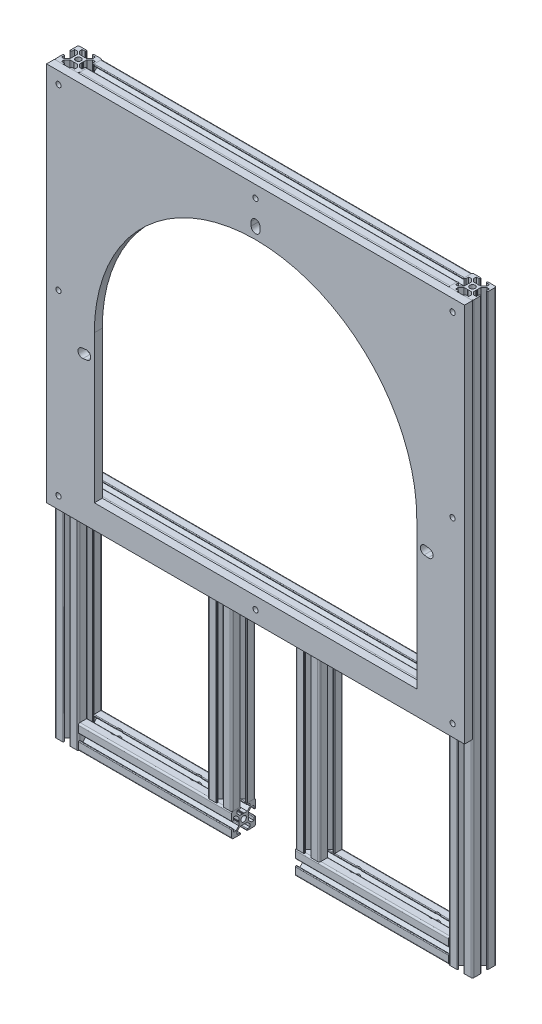
from build123d import *

# Parameters (mm, degrees)
F_30_X_30_X_R2_1_DEPTH      = 722.5
F_30_X_30_X_R2_1_DEPTH_BACK = 15
SKETCH_1_R                  = 3.4
SKETCH_1_ON_SEGMENT_2_R     = 3.4
F_30_X_30_X_R2_1_2_DEPTH    = 737.5
SKETCH_1_ON_SEGMENT_3_R     = 3.4
F_30_X_30_X_R2_1_3_DEPTH    = 497
SKETCH_1_ON_SEGMENT_4_R     = 3.4
F_30_X_30_X_R2_1_4_DEPTH    = 208.5
SKETCH_1_ON_SEGMENT_5_R     = 3.4
F_30_X_30_X_R2_1_5_DEPTH    = 497
SKETCH_1_ON_SEGMENT_6_R     = 3.4
F_30_X_30_X_R2_1_6_DEPTH    = 208.5
SKETCH_1_ON_SEGMENT_7_R     = 3.4
F_30_X_30_X_R2_1_7_DEPTH    = 262
SKETCH_1_ON_SEGMENT_8_R     = 3.4
F_30_X_30_X_R2_1_8_DEPTH    = 262
SKETCH_5_W                  = 525
SKETCH_5_H                  = 477.5
EXTRUDE_1_DEPTH             = 10
CUT_EXTRUDE_1_DEPTH         = 10
SKETCH_7_R                  = 3.25
CUT_EXTRUDE_2_DEPTH         = 10
SKETCH_8_R                  = 5.5
CUT_EXTRUDE_3_DEPTH         = 756.041389594


with BuildPart() as part:
    # 草图1 → 铝型材 30 X 30 X R2(1) (new, two sides: drawn at the far end of the back side and taken through both)
    with BuildSketch(Plane(origin=(-247.5, 367.5, 0), x_dir=(1, 0, 0), z_dir=(0, -1, 0)).offset(-F_30_X_30_X_R2_1_DEPTH_BACK)):
        with BuildLine():
            Line((-15, -4.8), (-15, -13))
            ThreePointArc((-15, -13), (-14.414213562, -14.414213562), (-13, -15))
            Line((-13, -15), (-4.8, -15))
            ThreePointArc((-4.8, -15), (-4.234314575, -14.765685425), (-4, -14.2))
            Line((-4, -14.2), (-4, -13.8))
            ThreePointArc((-4, -13.8), (-4.234314575, -13.234314575), (-4.8, -13))
            Line((-4.8, -13), (-8.25, -13))
            Line((-8.25, -13), (-8.25, -9.664213562))
            Line((-8.25, -9.664213562), (-4.585786438, -6))
            Line((-4.585786438, -6), (-0.653589838, -6))
            ThreePointArc((-0.653589838, -6), (-0.524180316, -5.982962913), (-0.403589838, -5.933012702))
            Line((-0.403589838, -5.933012702), (0, -5.7))
            Line((0, -5.7), (0.403589838, -5.933012702))
            ThreePointArc((0.403589838, -5.933012702), (0.653589838, -6), (0.903589838, -5.933012702))
            Line((0.903589838, -5.933012702), (1.218885629, -5.750976592))
            Line((1.218885629, -5.750976592), (2.5, -6))
            Line((2.5, -6), (4.585786438, -6))
            Line((4.585786438, -6), (8.25, -9.664213562))
            Line((8.25, -9.664213562), (8.25, -13))
            Line((8.25, -13), (4.8, -13))
            ThreePointArc((4.8, -13), (4.234314575, -13.234314575), (4, -13.8))
            Line((4, -13.8), (4, -14.2))
            ThreePointArc((4, -14.2), (4.234314575, -14.765685425), (4.8, -15))
            Line((4.8, -15), (13, -15))
            ThreePointArc((13, -15), (14.414213562, -14.414213562), (15, -13))
            Line((15, -13), (15, -4.8))
            ThreePointArc((15, -4.8), (14.765685425, -4.234314575), (14.2, -4))
            Line((14.2, -4), (13.8, -4))
            ThreePointArc((13.8, -4), (13.234314575, -4.234314575), (13, -4.8))
            Line((13, -4.8), (13, -8.25))
            Line((13, -8.25), (9.664213562, -8.25))
            Line((9.664213562, -8.25), (6, -4.585786438))
            Line((6, -4.585786438), (6, -0.653589838))
            ThreePointArc((6, -0.653589838), (5.982962913, -0.524180316), (5.933012702, -0.403589838))
            Line((5.933012702, -0.403589838), (5.7, 0))
            Line((5.7, 0), (5.933012702, 0.403589838))
            ThreePointArc((5.933012702, 0.403589838), (6, 0.653589838), (5.933012702, 0.903589838))
            Line((5.933012702, 0.903589838), (5.750976592, 1.218885629))
            Line((5.750976592, 1.218885629), (6, 2.5))
            Line((6, 2.5), (6, 4.585786438))
            Line((6, 4.585786438), (9.664213562, 8.25))
            Line((9.664213562, 8.25), (13, 8.25))
            Line((13, 8.25), (13, 4.8))
            ThreePointArc((13, 4.8), (13.234314575, 4.234314575), (13.8, 4))
            Line((13.8, 4), (14.2, 4))
            ThreePointArc((14.2, 4), (14.765685425, 4.234314575), (15, 4.8))
            Line((15, 4.8), (15, 13))
            ThreePointArc((15, 13), (14.414213562, 14.414213562), (13, 15))
            Line((13, 15), (4.8, 15))
            ThreePointArc((4.8, 15), (4.234314575, 14.765685425), (4, 14.2))
            Line((4, 14.2), (4, 13.8))
            ThreePointArc((4, 13.8), (4.234314575, 13.234314575), (4.8, 13))
            Line((4.8, 13), (8.25, 13))
            Line((8.25, 13), (8.25, 9.664213562))
            Line((8.25, 9.664213562), (4.585786438, 6))
            Line((4.585786438, 6), (0.653589838, 6))
            ThreePointArc((0.653589838, 6), (0.524180316, 5.982962913), (0.403589838, 5.933012702))
            Line((0.403589838, 5.933012702), (0, 5.7))
            Line((0, 5.7), (-0.403589838, 5.933012702))
            ThreePointArc((-0.403589838, 5.933012702), (-0.653589838, 6), (-0.903589838, 5.933012702))
            Line((-0.903589838, 5.933012702), (-1.218885629, 5.750976592))
            Line((-1.218885629, 5.750976592), (-2.5, 6))
            Line((-2.5, 6), (-4.585786438, 6))
            Line((-4.585786438, 6), (-8.25, 9.664213562))
            Line((-8.25, 9.664213562), (-8.25, 13))
            Line((-8.25, 13), (-4.8, 13))
            ThreePointArc((-4.8, 13), (-4.234314575, 13.234314575), (-4, 13.8))
            Line((-4, 13.8), (-4, 14.2))
            ThreePointArc((-4, 14.2), (-4.234314575, 14.765685425), (-4.8, 15))
            Line((-4.8, 15), (-13, 15))
            ThreePointArc((-13, 15), (-14.414213562, 14.414213562), (-15, 13))
            Line((-15, 13), (-15, 4.8))
            ThreePointArc((-15, 4.8), (-14.765685425, 4.234314575), (-14.2, 4))
            Line((-14.2, 4), (-13.8, 4))
            ThreePointArc((-13.8, 4), (-13.234314575, 4.234314575), (-13, 4.8))
            Line((-13, 4.8), (-13, 8.25))
            Line((-13, 8.25), (-9.664213562, 8.25))
            Line((-9.664213562, 8.25), (-6, 4.585786438))
            Line((-6, 4.585786438), (-6, 0.653589838))
            ThreePointArc((-6, 0.653589838), (-5.982962913, 0.524180316), (-5.933012702, 0.403589838))
            Line((-5.933012702, 0.403589838), (-5.7, 0))
            Line((-5.7, 0), (-5.933012702, -0.403589838))
            ThreePointArc((-5.933012702, -0.403589838), (-6, -0.653589838), (-5.933012702, -0.903589838))
            Line((-5.933012702, -0.903589838), (-5.750976592, -1.218885629))
            Line((-5.750976592, -1.218885629), (-6, -2.5))
            Line((-6, -2.5), (-6, -4.585786438))
            Line((-6, -4.585786438), (-9.664213562, -8.25))
            Line((-9.664213562, -8.25), (-13, -8.25))
            Line((-13, -8.25), (-13, -4.8))
            ThreePointArc((-13, -4.8), (-13.234314575, -4.234314575), (-13.8, -4))
            Line((-13.8, -4), (-14.2, -4))
            ThreePointArc((-14.2, -4), (-14.765685425, -4.234314575), (-15, -4.8))
        make_face()
        Circle(SKETCH_1_R, mode=Mode.SUBTRACT)
    extrude(amount=F_30_X_30_X_R2_1_DEPTH + F_30_X_30_X_R2_1_DEPTH_BACK)


with BuildPart() as body_2:
    # 草图1 on segment 2 (carried to segment 2) → 30 X 30 X R2_1 2 (new body)
    with BuildSketch(Plane(origin=(247.5, 382.5, 0), x_dir=(1, 0, 0), z_dir=(0, -1, 0))):
        with BuildLine():
            Line((-15, -4.8), (-15, -13))
            ThreePointArc((-15, -13), (-14.414213562, -14.414213562), (-13, -15))
            Line((-13, -15), (-4.8, -15))
            ThreePointArc((-4.8, -15), (-4.234314575, -14.765685425), (-4, -14.2))
            Line((-4, -14.2), (-4, -13.8))
            ThreePointArc((-4, -13.8), (-4.234314575, -13.234314575), (-4.8, -13))
            Line((-4.8, -13), (-8.25, -13))
            Line((-8.25, -13), (-8.25, -9.664213562))
            Line((-8.25, -9.664213562), (-4.585786438, -6))
            Line((-4.585786438, -6), (-0.653589838, -6))
            ThreePointArc((-0.653589838, -6), (-0.524180316, -5.982962913), (-0.403589838, -5.933012702))
            Line((-0.403589838, -5.933012702), (0, -5.7))
            Line((0, -5.7), (0.403589838, -5.933012702))
            ThreePointArc((0.403589838, -5.933012702), (0.653589838, -6), (0.903589838, -5.933012702))
            Line((0.903589838, -5.933012702), (1.218885629, -5.750976592))
            Line((1.218885629, -5.750976592), (2.5, -6))
            Line((2.5, -6), (4.585786438, -6))
            Line((4.585786438, -6), (8.25, -9.664213562))
            Line((8.25, -9.664213562), (8.25, -13))
            Line((8.25, -13), (4.8, -13))
            ThreePointArc((4.8, -13), (4.234314575, -13.234314575), (4, -13.8))
            Line((4, -13.8), (4, -14.2))
            ThreePointArc((4, -14.2), (4.234314575, -14.765685425), (4.8, -15))
            Line((4.8, -15), (13, -15))
            ThreePointArc((13, -15), (14.414213562, -14.414213562), (15, -13))
            Line((15, -13), (15, -4.8))
            ThreePointArc((15, -4.8), (14.765685425, -4.234314575), (14.2, -4))
            Line((14.2, -4), (13.8, -4))
            ThreePointArc((13.8, -4), (13.234314575, -4.234314575), (13, -4.8))
            Line((13, -4.8), (13, -8.25))
            Line((13, -8.25), (9.664213562, -8.25))
            Line((9.664213562, -8.25), (6, -4.585786438))
            Line((6, -4.585786438), (6, -0.653589838))
            ThreePointArc((6, -0.653589838), (5.982962913, -0.524180316), (5.933012702, -0.403589838))
            Line((5.933012702, -0.403589838), (5.7, 0))
            Line((5.7, 0), (5.933012702, 0.403589838))
            ThreePointArc((5.933012702, 0.403589838), (6, 0.653589838), (5.933012702, 0.903589838))
            Line((5.933012702, 0.903589838), (5.750976592, 1.218885629))
            Line((5.750976592, 1.218885629), (6, 2.5))
            Line((6, 2.5), (6, 4.585786438))
            Line((6, 4.585786438), (9.664213562, 8.25))
            Line((9.664213562, 8.25), (13, 8.25))
            Line((13, 8.25), (13, 4.8))
            ThreePointArc((13, 4.8), (13.234314575, 4.234314575), (13.8, 4))
            Line((13.8, 4), (14.2, 4))
            ThreePointArc((14.2, 4), (14.765685425, 4.234314575), (15, 4.8))
            Line((15, 4.8), (15, 13))
            ThreePointArc((15, 13), (14.414213562, 14.414213562), (13, 15))
            Line((13, 15), (4.8, 15))
            ThreePointArc((4.8, 15), (4.234314575, 14.765685425), (4, 14.2))
            Line((4, 14.2), (4, 13.8))
            ThreePointArc((4, 13.8), (4.234314575, 13.234314575), (4.8, 13))
            Line((4.8, 13), (8.25, 13))
            Line((8.25, 13), (8.25, 9.664213562))
            Line((8.25, 9.664213562), (4.585786438, 6))
            Line((4.585786438, 6), (0.653589838, 6))
            ThreePointArc((0.653589838, 6), (0.524180316, 5.982962913), (0.403589838, 5.933012702))
            Line((0.403589838, 5.933012702), (0, 5.7))
            Line((0, 5.7), (-0.403589838, 5.933012702))
            ThreePointArc((-0.403589838, 5.933012702), (-0.653589838, 6), (-0.903589838, 5.933012702))
            Line((-0.903589838, 5.933012702), (-1.218885629, 5.750976592))
            Line((-1.218885629, 5.750976592), (-2.5, 6))
            Line((-2.5, 6), (-4.585786438, 6))
            Line((-4.585786438, 6), (-8.25, 9.664213562))
            Line((-8.25, 9.664213562), (-8.25, 13))
            Line((-8.25, 13), (-4.8, 13))
            ThreePointArc((-4.8, 13), (-4.234314575, 13.234314575), (-4, 13.8))
            Line((-4, 13.8), (-4, 14.2))
            ThreePointArc((-4, 14.2), (-4.234314575, 14.765685425), (-4.8, 15))
            Line((-4.8, 15), (-13, 15))
            ThreePointArc((-13, 15), (-14.414213562, 14.414213562), (-15, 13))
            Line((-15, 13), (-15, 4.8))
            ThreePointArc((-15, 4.8), (-14.765685425, 4.234314575), (-14.2, 4))
            Line((-14.2, 4), (-13.8, 4))
            ThreePointArc((-13.8, 4), (-13.234314575, 4.234314575), (-13, 4.8))
            Line((-13, 4.8), (-13, 8.25))
            Line((-13, 8.25), (-9.664213562, 8.25))
            Line((-9.664213562, 8.25), (-6, 4.585786438))
            Line((-6, 4.585786438), (-6, 0.653589838))
            ThreePointArc((-6, 0.653589838), (-5.982962913, 0.524180316), (-5.933012702, 0.403589838))
            Line((-5.933012702, 0.403589838), (-5.7, 0))
            Line((-5.7, 0), (-5.933012702, -0.403589838))
            ThreePointArc((-5.933012702, -0.403589838), (-6, -0.653589838), (-5.933012702, -0.903589838))
            Line((-5.933012702, -0.903589838), (-5.750976592, -1.218885629))
            Line((-5.750976592, -1.218885629), (-6, -2.5))
            Line((-6, -2.5), (-6, -4.585786438))
            Line((-6, -4.585786438), (-9.664213562, -8.25))
            Line((-9.664213562, -8.25), (-13, -8.25))
            Line((-13, -8.25), (-13, -4.8))
            ThreePointArc((-13, -4.8), (-13.234314575, -4.234314575), (-13.8, -4))
            Line((-13.8, -4), (-14.2, -4))
            ThreePointArc((-14.2, -4), (-14.765685425, -4.234314575), (-15, -4.8))
        make_face()
        Circle(SKETCH_1_ON_SEGMENT_2_R, mode=Mode.SUBTRACT)
    extrude(amount=F_30_X_30_X_R2_1_2_DEPTH)


with BuildPart() as body_3:
    # 草图1 on segment 3 (carried to segment 3) → 30 X 30 X R2_1 3 (new body)
    with BuildSketch(Plane(origin=(-248.5, 367.5, 0), x_dir=(0, 1, 0), z_dir=(1, 0, 0))):
        with BuildLine():
            Line((-15, -4.8), (-15, -13))
            ThreePointArc((-15, -13), (-14.414213562, -14.414213562), (-13, -15))
            Line((-13, -15), (-4.8, -15))
            ThreePointArc((-4.8, -15), (-4.234314575, -14.765685425), (-4, -14.2))
            Line((-4, -14.2), (-4, -13.8))
            ThreePointArc((-4, -13.8), (-4.234314575, -13.234314575), (-4.8, -13))
            Line((-4.8, -13), (-8.25, -13))
            Line((-8.25, -13), (-8.25, -9.664213562))
            Line((-8.25, -9.664213562), (-4.585786438, -6))
            Line((-4.585786438, -6), (-0.653589838, -6))
            ThreePointArc((-0.653589838, -6), (-0.524180316, -5.982962913), (-0.403589838, -5.933012702))
            Line((-0.403589838, -5.933012702), (0, -5.7))
            Line((0, -5.7), (0.403589838, -5.933012702))
            ThreePointArc((0.403589838, -5.933012702), (0.653589838, -6), (0.903589838, -5.933012702))
            Line((0.903589838, -5.933012702), (1.218885629, -5.750976592))
            Line((1.218885629, -5.750976592), (2.5, -6))
            Line((2.5, -6), (4.585786438, -6))
            Line((4.585786438, -6), (8.25, -9.664213562))
            Line((8.25, -9.664213562), (8.25, -13))
            Line((8.25, -13), (4.8, -13))
            ThreePointArc((4.8, -13), (4.234314575, -13.234314575), (4, -13.8))
            Line((4, -13.8), (4, -14.2))
            ThreePointArc((4, -14.2), (4.234314575, -14.765685425), (4.8, -15))
            Line((4.8, -15), (13, -15))
            ThreePointArc((13, -15), (14.414213562, -14.414213562), (15, -13))
            Line((15, -13), (15, -4.8))
            ThreePointArc((15, -4.8), (14.765685425, -4.234314575), (14.2, -4))
            Line((14.2, -4), (13.8, -4))
            ThreePointArc((13.8, -4), (13.234314575, -4.234314575), (13, -4.8))
            Line((13, -4.8), (13, -8.25))
            Line((13, -8.25), (9.664213562, -8.25))
            Line((9.664213562, -8.25), (6, -4.585786438))
            Line((6, -4.585786438), (6, -0.653589838))
            ThreePointArc((6, -0.653589838), (5.982962913, -0.524180316), (5.933012702, -0.403589838))
            Line((5.933012702, -0.403589838), (5.7, 0))
            Line((5.7, 0), (5.933012702, 0.403589838))
            ThreePointArc((5.933012702, 0.403589838), (6, 0.653589838), (5.933012702, 0.903589838))
            Line((5.933012702, 0.903589838), (5.750976592, 1.218885629))
            Line((5.750976592, 1.218885629), (6, 2.5))
            Line((6, 2.5), (6, 4.585786438))
            Line((6, 4.585786438), (9.664213562, 8.25))
            Line((9.664213562, 8.25), (13, 8.25))
            Line((13, 8.25), (13, 4.8))
            ThreePointArc((13, 4.8), (13.234314575, 4.234314575), (13.8, 4))
            Line((13.8, 4), (14.2, 4))
            ThreePointArc((14.2, 4), (14.765685425, 4.234314575), (15, 4.8))
            Line((15, 4.8), (15, 13))
            ThreePointArc((15, 13), (14.414213562, 14.414213562), (13, 15))
            Line((13, 15), (4.8, 15))
            ThreePointArc((4.8, 15), (4.234314575, 14.765685425), (4, 14.2))
            Line((4, 14.2), (4, 13.8))
            ThreePointArc((4, 13.8), (4.234314575, 13.234314575), (4.8, 13))
            Line((4.8, 13), (8.25, 13))
            Line((8.25, 13), (8.25, 9.664213562))
            Line((8.25, 9.664213562), (4.585786438, 6))
            Line((4.585786438, 6), (0.653589838, 6))
            ThreePointArc((0.653589838, 6), (0.524180316, 5.982962913), (0.403589838, 5.933012702))
            Line((0.403589838, 5.933012702), (0, 5.7))
            Line((0, 5.7), (-0.403589838, 5.933012702))
            ThreePointArc((-0.403589838, 5.933012702), (-0.653589838, 6), (-0.903589838, 5.933012702))
            Line((-0.903589838, 5.933012702), (-1.218885629, 5.750976592))
            Line((-1.218885629, 5.750976592), (-2.5, 6))
            Line((-2.5, 6), (-4.585786438, 6))
            Line((-4.585786438, 6), (-8.25, 9.664213562))
            Line((-8.25, 9.664213562), (-8.25, 13))
            Line((-8.25, 13), (-4.8, 13))
            ThreePointArc((-4.8, 13), (-4.234314575, 13.234314575), (-4, 13.8))
            Line((-4, 13.8), (-4, 14.2))
            ThreePointArc((-4, 14.2), (-4.234314575, 14.765685425), (-4.8, 15))
            Line((-4.8, 15), (-13, 15))
            ThreePointArc((-13, 15), (-14.414213562, 14.414213562), (-15, 13))
            Line((-15, 13), (-15, 4.8))
            ThreePointArc((-15, 4.8), (-14.765685425, 4.234314575), (-14.2, 4))
            Line((-14.2, 4), (-13.8, 4))
            ThreePointArc((-13.8, 4), (-13.234314575, 4.234314575), (-13, 4.8))
            Line((-13, 4.8), (-13, 8.25))
            Line((-13, 8.25), (-9.664213562, 8.25))
            Line((-9.664213562, 8.25), (-6, 4.585786438))
            Line((-6, 4.585786438), (-6, 0.653589838))
            ThreePointArc((-6, 0.653589838), (-5.982962913, 0.524180316), (-5.933012702, 0.403589838))
            Line((-5.933012702, 0.403589838), (-5.7, 0))
            Line((-5.7, 0), (-5.933012702, -0.403589838))
            ThreePointArc((-5.933012702, -0.403589838), (-6, -0.653589838), (-5.933012702, -0.903589838))
            Line((-5.933012702, -0.903589838), (-5.750976592, -1.218885629))
            Line((-5.750976592, -1.218885629), (-6, -2.5))
            Line((-6, -2.5), (-6, -4.585786438))
            Line((-6, -4.585786438), (-9.664213562, -8.25))
            Line((-9.664213562, -8.25), (-13, -8.25))
            Line((-13, -8.25), (-13, -4.8))
            ThreePointArc((-13, -4.8), (-13.234314575, -4.234314575), (-13.8, -4))
            Line((-13.8, -4), (-14.2, -4))
            ThreePointArc((-14.2, -4), (-14.765685425, -4.234314575), (-15, -4.8))
        make_face()
        Circle(SKETCH_1_ON_SEGMENT_3_R, mode=Mode.SUBTRACT)
    extrude(amount=F_30_X_30_X_R2_1_3_DEPTH)

    # 30 X 30 X R2_1 3 end butt 1
    split(bisect_by=Plane(origin=(-232.5, 367.5, 0), x_dir=(0, 1, 0), z_dir=(1, 0, 0)), keep=Keep.TOP)

    # 30 X 30 X R2_1 3 end butt 2
    split(bisect_by=Plane(origin=(232.5, 367.5, 0), x_dir=(0, -1, 0), z_dir=(-1, 0, 0)), keep=Keep.TOP)


with BuildPart() as body_4:
    # 草图1 on segment 4 (carried to segment 4) → 30 X 30 X R2_1 4 (new body)
    with BuildSketch(Plane(origin=(-248.5, -340, 0), x_dir=(0, 1, 0), z_dir=(1, 0, 0))):
        with BuildLine():
            Line((-15, -4.8), (-15, -13))
            ThreePointArc((-15, -13), (-14.414213562, -14.414213562), (-13, -15))
            Line((-13, -15), (-4.8, -15))
            ThreePointArc((-4.8, -15), (-4.234314575, -14.765685425), (-4, -14.2))
            Line((-4, -14.2), (-4, -13.8))
            ThreePointArc((-4, -13.8), (-4.234314575, -13.234314575), (-4.8, -13))
            Line((-4.8, -13), (-8.25, -13))
            Line((-8.25, -13), (-8.25, -9.664213562))
            Line((-8.25, -9.664213562), (-4.585786438, -6))
            Line((-4.585786438, -6), (-0.653589838, -6))
            ThreePointArc((-0.653589838, -6), (-0.524180316, -5.982962913), (-0.403589838, -5.933012702))
            Line((-0.403589838, -5.933012702), (0, -5.7))
            Line((0, -5.7), (0.403589838, -5.933012702))
            ThreePointArc((0.403589838, -5.933012702), (0.653589838, -6), (0.903589838, -5.933012702))
            Line((0.903589838, -5.933012702), (1.218885629, -5.750976592))
            Line((1.218885629, -5.750976592), (2.5, -6))
            Line((2.5, -6), (4.585786438, -6))
            Line((4.585786438, -6), (8.25, -9.664213562))
            Line((8.25, -9.664213562), (8.25, -13))
            Line((8.25, -13), (4.8, -13))
            ThreePointArc((4.8, -13), (4.234314575, -13.234314575), (4, -13.8))
            Line((4, -13.8), (4, -14.2))
            ThreePointArc((4, -14.2), (4.234314575, -14.765685425), (4.8, -15))
            Line((4.8, -15), (13, -15))
            ThreePointArc((13, -15), (14.414213562, -14.414213562), (15, -13))
            Line((15, -13), (15, -4.8))
            ThreePointArc((15, -4.8), (14.765685425, -4.234314575), (14.2, -4))
            Line((14.2, -4), (13.8, -4))
            ThreePointArc((13.8, -4), (13.234314575, -4.234314575), (13, -4.8))
            Line((13, -4.8), (13, -8.25))
            Line((13, -8.25), (9.664213562, -8.25))
            Line((9.664213562, -8.25), (6, -4.585786438))
            Line((6, -4.585786438), (6, -0.653589838))
            ThreePointArc((6, -0.653589838), (5.982962913, -0.524180316), (5.933012702, -0.403589838))
            Line((5.933012702, -0.403589838), (5.7, 0))
            Line((5.7, 0), (5.933012702, 0.403589838))
            ThreePointArc((5.933012702, 0.403589838), (6, 0.653589838), (5.933012702, 0.903589838))
            Line((5.933012702, 0.903589838), (5.750976592, 1.218885629))
            Line((5.750976592, 1.218885629), (6, 2.5))
            Line((6, 2.5), (6, 4.585786438))
            Line((6, 4.585786438), (9.664213562, 8.25))
            Line((9.664213562, 8.25), (13, 8.25))
            Line((13, 8.25), (13, 4.8))
            ThreePointArc((13, 4.8), (13.234314575, 4.234314575), (13.8, 4))
            Line((13.8, 4), (14.2, 4))
            ThreePointArc((14.2, 4), (14.765685425, 4.234314575), (15, 4.8))
            Line((15, 4.8), (15, 13))
            ThreePointArc((15, 13), (14.414213562, 14.414213562), (13, 15))
            Line((13, 15), (4.8, 15))
            ThreePointArc((4.8, 15), (4.234314575, 14.765685425), (4, 14.2))
            Line((4, 14.2), (4, 13.8))
            ThreePointArc((4, 13.8), (4.234314575, 13.234314575), (4.8, 13))
            Line((4.8, 13), (8.25, 13))
            Line((8.25, 13), (8.25, 9.664213562))
            Line((8.25, 9.664213562), (4.585786438, 6))
            Line((4.585786438, 6), (0.653589838, 6))
            ThreePointArc((0.653589838, 6), (0.524180316, 5.982962913), (0.403589838, 5.933012702))
            Line((0.403589838, 5.933012702), (0, 5.7))
            Line((0, 5.7), (-0.403589838, 5.933012702))
            ThreePointArc((-0.403589838, 5.933012702), (-0.653589838, 6), (-0.903589838, 5.933012702))
            Line((-0.903589838, 5.933012702), (-1.218885629, 5.750976592))
            Line((-1.218885629, 5.750976592), (-2.5, 6))
            Line((-2.5, 6), (-4.585786438, 6))
            Line((-4.585786438, 6), (-8.25, 9.664213562))
            Line((-8.25, 9.664213562), (-8.25, 13))
            Line((-8.25, 13), (-4.8, 13))
            ThreePointArc((-4.8, 13), (-4.234314575, 13.234314575), (-4, 13.8))
            Line((-4, 13.8), (-4, 14.2))
            ThreePointArc((-4, 14.2), (-4.234314575, 14.765685425), (-4.8, 15))
            Line((-4.8, 15), (-13, 15))
            ThreePointArc((-13, 15), (-14.414213562, 14.414213562), (-15, 13))
            Line((-15, 13), (-15, 4.8))
            ThreePointArc((-15, 4.8), (-14.765685425, 4.234314575), (-14.2, 4))
            Line((-14.2, 4), (-13.8, 4))
            ThreePointArc((-13.8, 4), (-13.234314575, 4.234314575), (-13, 4.8))
            Line((-13, 4.8), (-13, 8.25))
            Line((-13, 8.25), (-9.664213562, 8.25))
            Line((-9.664213562, 8.25), (-6, 4.585786438))
            Line((-6, 4.585786438), (-6, 0.653589838))
            ThreePointArc((-6, 0.653589838), (-5.982962913, 0.524180316), (-5.933012702, 0.403589838))
            Line((-5.933012702, 0.403589838), (-5.7, 0))
            Line((-5.7, 0), (-5.933012702, -0.403589838))
            ThreePointArc((-5.933012702, -0.403589838), (-6, -0.653589838), (-5.933012702, -0.903589838))
            Line((-5.933012702, -0.903589838), (-5.750976592, -1.218885629))
            Line((-5.750976592, -1.218885629), (-6, -2.5))
            Line((-6, -2.5), (-6, -4.585786438))
            Line((-6, -4.585786438), (-9.664213562, -8.25))
            Line((-9.664213562, -8.25), (-13, -8.25))
            Line((-13, -8.25), (-13, -4.8))
            ThreePointArc((-13, -4.8), (-13.234314575, -4.234314575), (-13.8, -4))
            Line((-13.8, -4), (-14.2, -4))
            ThreePointArc((-14.2, -4), (-14.765685425, -4.234314575), (-15, -4.8))
        make_face()
        Circle(SKETCH_1_ON_SEGMENT_4_R, mode=Mode.SUBTRACT)
    extrude(amount=F_30_X_30_X_R2_1_4_DEPTH)

    # 30 X 30 X R2_1 4 end butt 1
    split(bisect_by=Plane(origin=(-232.5, -340, 0), x_dir=(0, 1, 0), z_dir=(1, 0, 0)), keep=Keep.TOP)


with BuildPart() as body_5:
    # 草图1 on segment 5 (carried to segment 5) → 30 X 30 X R2_1 5 (new body)
    with BuildSketch(Plane(origin=(-248.5, -80, 0), x_dir=(0, 1, 0), z_dir=(1, 0, 0))):
        with BuildLine():
            Line((-15, -4.8), (-15, -13))
            ThreePointArc((-15, -13), (-14.414213562, -14.414213562), (-13, -15))
            Line((-13, -15), (-4.8, -15))
            ThreePointArc((-4.8, -15), (-4.234314575, -14.765685425), (-4, -14.2))
            Line((-4, -14.2), (-4, -13.8))
            ThreePointArc((-4, -13.8), (-4.234314575, -13.234314575), (-4.8, -13))
            Line((-4.8, -13), (-8.25, -13))
            Line((-8.25, -13), (-8.25, -9.664213562))
            Line((-8.25, -9.664213562), (-4.585786438, -6))
            Line((-4.585786438, -6), (-0.653589838, -6))
            ThreePointArc((-0.653589838, -6), (-0.524180316, -5.982962913), (-0.403589838, -5.933012702))
            Line((-0.403589838, -5.933012702), (0, -5.7))
            Line((0, -5.7), (0.403589838, -5.933012702))
            ThreePointArc((0.403589838, -5.933012702), (0.653589838, -6), (0.903589838, -5.933012702))
            Line((0.903589838, -5.933012702), (1.218885629, -5.750976592))
            Line((1.218885629, -5.750976592), (2.5, -6))
            Line((2.5, -6), (4.585786438, -6))
            Line((4.585786438, -6), (8.25, -9.664213562))
            Line((8.25, -9.664213562), (8.25, -13))
            Line((8.25, -13), (4.8, -13))
            ThreePointArc((4.8, -13), (4.234314575, -13.234314575), (4, -13.8))
            Line((4, -13.8), (4, -14.2))
            ThreePointArc((4, -14.2), (4.234314575, -14.765685425), (4.8, -15))
            Line((4.8, -15), (13, -15))
            ThreePointArc((13, -15), (14.414213562, -14.414213562), (15, -13))
            Line((15, -13), (15, -4.8))
            ThreePointArc((15, -4.8), (14.765685425, -4.234314575), (14.2, -4))
            Line((14.2, -4), (13.8, -4))
            ThreePointArc((13.8, -4), (13.234314575, -4.234314575), (13, -4.8))
            Line((13, -4.8), (13, -8.25))
            Line((13, -8.25), (9.664213562, -8.25))
            Line((9.664213562, -8.25), (6, -4.585786438))
            Line((6, -4.585786438), (6, -0.653589838))
            ThreePointArc((6, -0.653589838), (5.982962913, -0.524180316), (5.933012702, -0.403589838))
            Line((5.933012702, -0.403589838), (5.7, 0))
            Line((5.7, 0), (5.933012702, 0.403589838))
            ThreePointArc((5.933012702, 0.403589838), (6, 0.653589838), (5.933012702, 0.903589838))
            Line((5.933012702, 0.903589838), (5.750976592, 1.218885629))
            Line((5.750976592, 1.218885629), (6, 2.5))
            Line((6, 2.5), (6, 4.585786438))
            Line((6, 4.585786438), (9.664213562, 8.25))
            Line((9.664213562, 8.25), (13, 8.25))
            Line((13, 8.25), (13, 4.8))
            ThreePointArc((13, 4.8), (13.234314575, 4.234314575), (13.8, 4))
            Line((13.8, 4), (14.2, 4))
            ThreePointArc((14.2, 4), (14.765685425, 4.234314575), (15, 4.8))
            Line((15, 4.8), (15, 13))
            ThreePointArc((15, 13), (14.414213562, 14.414213562), (13, 15))
            Line((13, 15), (4.8, 15))
            ThreePointArc((4.8, 15), (4.234314575, 14.765685425), (4, 14.2))
            Line((4, 14.2), (4, 13.8))
            ThreePointArc((4, 13.8), (4.234314575, 13.234314575), (4.8, 13))
            Line((4.8, 13), (8.25, 13))
            Line((8.25, 13), (8.25, 9.664213562))
            Line((8.25, 9.664213562), (4.585786438, 6))
            Line((4.585786438, 6), (0.653589838, 6))
            ThreePointArc((0.653589838, 6), (0.524180316, 5.982962913), (0.403589838, 5.933012702))
            Line((0.403589838, 5.933012702), (0, 5.7))
            Line((0, 5.7), (-0.403589838, 5.933012702))
            ThreePointArc((-0.403589838, 5.933012702), (-0.653589838, 6), (-0.903589838, 5.933012702))
            Line((-0.903589838, 5.933012702), (-1.218885629, 5.750976592))
            Line((-1.218885629, 5.750976592), (-2.5, 6))
            Line((-2.5, 6), (-4.585786438, 6))
            Line((-4.585786438, 6), (-8.25, 9.664213562))
            Line((-8.25, 9.664213562), (-8.25, 13))
            Line((-8.25, 13), (-4.8, 13))
            ThreePointArc((-4.8, 13), (-4.234314575, 13.234314575), (-4, 13.8))
            Line((-4, 13.8), (-4, 14.2))
            ThreePointArc((-4, 14.2), (-4.234314575, 14.765685425), (-4.8, 15))
            Line((-4.8, 15), (-13, 15))
            ThreePointArc((-13, 15), (-14.414213562, 14.414213562), (-15, 13))
            Line((-15, 13), (-15, 4.8))
            ThreePointArc((-15, 4.8), (-14.765685425, 4.234314575), (-14.2, 4))
            Line((-14.2, 4), (-13.8, 4))
            ThreePointArc((-13.8, 4), (-13.234314575, 4.234314575), (-13, 4.8))
            Line((-13, 4.8), (-13, 8.25))
            Line((-13, 8.25), (-9.664213562, 8.25))
            Line((-9.664213562, 8.25), (-6, 4.585786438))
            Line((-6, 4.585786438), (-6, 0.653589838))
            ThreePointArc((-6, 0.653589838), (-5.982962913, 0.524180316), (-5.933012702, 0.403589838))
            Line((-5.933012702, 0.403589838), (-5.7, 0))
            Line((-5.7, 0), (-5.933012702, -0.403589838))
            ThreePointArc((-5.933012702, -0.403589838), (-6, -0.653589838), (-5.933012702, -0.903589838))
            Line((-5.933012702, -0.903589838), (-5.750976592, -1.218885629))
            Line((-5.750976592, -1.218885629), (-6, -2.5))
            Line((-6, -2.5), (-6, -4.585786438))
            Line((-6, -4.585786438), (-9.664213562, -8.25))
            Line((-9.664213562, -8.25), (-13, -8.25))
            Line((-13, -8.25), (-13, -4.8))
            ThreePointArc((-13, -4.8), (-13.234314575, -4.234314575), (-13.8, -4))
            Line((-13.8, -4), (-14.2, -4))
            ThreePointArc((-14.2, -4), (-14.765685425, -4.234314575), (-15, -4.8))
        make_face()
        Circle(SKETCH_1_ON_SEGMENT_5_R, mode=Mode.SUBTRACT)
    extrude(amount=F_30_X_30_X_R2_1_5_DEPTH)

    # 30 X 30 X R2_1 5 end butt 1
    split(bisect_by=Plane(origin=(-232.5, -80, 0), x_dir=(0, 1, 0), z_dir=(1, 0, 0)), keep=Keep.TOP)

    # 30 X 30 X R2_1 5 end butt 2
    split(bisect_by=Plane(origin=(232.5, -80, 0), x_dir=(0, -1, 0), z_dir=(-1, 0, 0)), keep=Keep.TOP)


with BuildPart() as body_6:
    # 草图1 on segment 6 (carried to segment 6) → 30 X 30 X R2_1 6 (new body)
    with BuildSketch(Plane(origin=(40, -340, 0), x_dir=(0, 1, 0), z_dir=(1, 0, 0))):
        with BuildLine():
            Line((-15, -4.8), (-15, -13))
            ThreePointArc((-15, -13), (-14.414213562, -14.414213562), (-13, -15))
            Line((-13, -15), (-4.8, -15))
            ThreePointArc((-4.8, -15), (-4.234314575, -14.765685425), (-4, -14.2))
            Line((-4, -14.2), (-4, -13.8))
            ThreePointArc((-4, -13.8), (-4.234314575, -13.234314575), (-4.8, -13))
            Line((-4.8, -13), (-8.25, -13))
            Line((-8.25, -13), (-8.25, -9.664213562))
            Line((-8.25, -9.664213562), (-4.585786438, -6))
            Line((-4.585786438, -6), (-0.653589838, -6))
            ThreePointArc((-0.653589838, -6), (-0.524180316, -5.982962913), (-0.403589838, -5.933012702))
            Line((-0.403589838, -5.933012702), (0, -5.7))
            Line((0, -5.7), (0.403589838, -5.933012702))
            ThreePointArc((0.403589838, -5.933012702), (0.653589838, -6), (0.903589838, -5.933012702))
            Line((0.903589838, -5.933012702), (1.218885629, -5.750976592))
            Line((1.218885629, -5.750976592), (2.5, -6))
            Line((2.5, -6), (4.585786438, -6))
            Line((4.585786438, -6), (8.25, -9.664213562))
            Line((8.25, -9.664213562), (8.25, -13))
            Line((8.25, -13), (4.8, -13))
            ThreePointArc((4.8, -13), (4.234314575, -13.234314575), (4, -13.8))
            Line((4, -13.8), (4, -14.2))
            ThreePointArc((4, -14.2), (4.234314575, -14.765685425), (4.8, -15))
            Line((4.8, -15), (13, -15))
            ThreePointArc((13, -15), (14.414213562, -14.414213562), (15, -13))
            Line((15, -13), (15, -4.8))
            ThreePointArc((15, -4.8), (14.765685425, -4.234314575), (14.2, -4))
            Line((14.2, -4), (13.8, -4))
            ThreePointArc((13.8, -4), (13.234314575, -4.234314575), (13, -4.8))
            Line((13, -4.8), (13, -8.25))
            Line((13, -8.25), (9.664213562, -8.25))
            Line((9.664213562, -8.25), (6, -4.585786438))
            Line((6, -4.585786438), (6, -0.653589838))
            ThreePointArc((6, -0.653589838), (5.982962913, -0.524180316), (5.933012702, -0.403589838))
            Line((5.933012702, -0.403589838), (5.7, 0))
            Line((5.7, 0), (5.933012702, 0.403589838))
            ThreePointArc((5.933012702, 0.403589838), (6, 0.653589838), (5.933012702, 0.903589838))
            Line((5.933012702, 0.903589838), (5.750976592, 1.218885629))
            Line((5.750976592, 1.218885629), (6, 2.5))
            Line((6, 2.5), (6, 4.585786438))
            Line((6, 4.585786438), (9.664213562, 8.25))
            Line((9.664213562, 8.25), (13, 8.25))
            Line((13, 8.25), (13, 4.8))
            ThreePointArc((13, 4.8), (13.234314575, 4.234314575), (13.8, 4))
            Line((13.8, 4), (14.2, 4))
            ThreePointArc((14.2, 4), (14.765685425, 4.234314575), (15, 4.8))
            Line((15, 4.8), (15, 13))
            ThreePointArc((15, 13), (14.414213562, 14.414213562), (13, 15))
            Line((13, 15), (4.8, 15))
            ThreePointArc((4.8, 15), (4.234314575, 14.765685425), (4, 14.2))
            Line((4, 14.2), (4, 13.8))
            ThreePointArc((4, 13.8), (4.234314575, 13.234314575), (4.8, 13))
            Line((4.8, 13), (8.25, 13))
            Line((8.25, 13), (8.25, 9.664213562))
            Line((8.25, 9.664213562), (4.585786438, 6))
            Line((4.585786438, 6), (0.653589838, 6))
            ThreePointArc((0.653589838, 6), (0.524180316, 5.982962913), (0.403589838, 5.933012702))
            Line((0.403589838, 5.933012702), (0, 5.7))
            Line((0, 5.7), (-0.403589838, 5.933012702))
            ThreePointArc((-0.403589838, 5.933012702), (-0.653589838, 6), (-0.903589838, 5.933012702))
            Line((-0.903589838, 5.933012702), (-1.218885629, 5.750976592))
            Line((-1.218885629, 5.750976592), (-2.5, 6))
            Line((-2.5, 6), (-4.585786438, 6))
            Line((-4.585786438, 6), (-8.25, 9.664213562))
            Line((-8.25, 9.664213562), (-8.25, 13))
            Line((-8.25, 13), (-4.8, 13))
            ThreePointArc((-4.8, 13), (-4.234314575, 13.234314575), (-4, 13.8))
            Line((-4, 13.8), (-4, 14.2))
            ThreePointArc((-4, 14.2), (-4.234314575, 14.765685425), (-4.8, 15))
            Line((-4.8, 15), (-13, 15))
            ThreePointArc((-13, 15), (-14.414213562, 14.414213562), (-15, 13))
            Line((-15, 13), (-15, 4.8))
            ThreePointArc((-15, 4.8), (-14.765685425, 4.234314575), (-14.2, 4))
            Line((-14.2, 4), (-13.8, 4))
            ThreePointArc((-13.8, 4), (-13.234314575, 4.234314575), (-13, 4.8))
            Line((-13, 4.8), (-13, 8.25))
            Line((-13, 8.25), (-9.664213562, 8.25))
            Line((-9.664213562, 8.25), (-6, 4.585786438))
            Line((-6, 4.585786438), (-6, 0.653589838))
            ThreePointArc((-6, 0.653589838), (-5.982962913, 0.524180316), (-5.933012702, 0.403589838))
            Line((-5.933012702, 0.403589838), (-5.7, 0))
            Line((-5.7, 0), (-5.933012702, -0.403589838))
            ThreePointArc((-5.933012702, -0.403589838), (-6, -0.653589838), (-5.933012702, -0.903589838))
            Line((-5.933012702, -0.903589838), (-5.750976592, -1.218885629))
            Line((-5.750976592, -1.218885629), (-6, -2.5))
            Line((-6, -2.5), (-6, -4.585786438))
            Line((-6, -4.585786438), (-9.664213562, -8.25))
            Line((-9.664213562, -8.25), (-13, -8.25))
            Line((-13, -8.25), (-13, -4.8))
            ThreePointArc((-13, -4.8), (-13.234314575, -4.234314575), (-13.8, -4))
            Line((-13.8, -4), (-14.2, -4))
            ThreePointArc((-14.2, -4), (-14.765685425, -4.234314575), (-15, -4.8))
        make_face()
        Circle(SKETCH_1_ON_SEGMENT_6_R, mode=Mode.SUBTRACT)
    extrude(amount=F_30_X_30_X_R2_1_6_DEPTH)

    # 30 X 30 X R2_1 6 end butt 1
    split(bisect_by=Plane(origin=(232.5, -340, 0), x_dir=(0, -1, 0), z_dir=(-1, 0, 0)), keep=Keep.TOP)


with BuildPart() as body_7:
    # 草图1 on segment 7 (carried to segment 7) → 30 X 30 X R2_1 7 (new body)
    with BuildSketch(Plane(origin=(-55, -79, 0), x_dir=(1, 0, 0), z_dir=(0, -1, 0))):
        with BuildLine():
            Line((-15, -4.8), (-15, -13))
            ThreePointArc((-15, -13), (-14.414213562, -14.414213562), (-13, -15))
            Line((-13, -15), (-4.8, -15))
            ThreePointArc((-4.8, -15), (-4.234314575, -14.765685425), (-4, -14.2))
            Line((-4, -14.2), (-4, -13.8))
            ThreePointArc((-4, -13.8), (-4.234314575, -13.234314575), (-4.8, -13))
            Line((-4.8, -13), (-8.25, -13))
            Line((-8.25, -13), (-8.25, -9.664213562))
            Line((-8.25, -9.664213562), (-4.585786438, -6))
            Line((-4.585786438, -6), (-0.653589838, -6))
            ThreePointArc((-0.653589838, -6), (-0.524180316, -5.982962913), (-0.403589838, -5.933012702))
            Line((-0.403589838, -5.933012702), (0, -5.7))
            Line((0, -5.7), (0.403589838, -5.933012702))
            ThreePointArc((0.403589838, -5.933012702), (0.653589838, -6), (0.903589838, -5.933012702))
            Line((0.903589838, -5.933012702), (1.218885629, -5.750976592))
            Line((1.218885629, -5.750976592), (2.5, -6))
            Line((2.5, -6), (4.585786438, -6))
            Line((4.585786438, -6), (8.25, -9.664213562))
            Line((8.25, -9.664213562), (8.25, -13))
            Line((8.25, -13), (4.8, -13))
            ThreePointArc((4.8, -13), (4.234314575, -13.234314575), (4, -13.8))
            Line((4, -13.8), (4, -14.2))
            ThreePointArc((4, -14.2), (4.234314575, -14.765685425), (4.8, -15))
            Line((4.8, -15), (13, -15))
            ThreePointArc((13, -15), (14.414213562, -14.414213562), (15, -13))
            Line((15, -13), (15, -4.8))
            ThreePointArc((15, -4.8), (14.765685425, -4.234314575), (14.2, -4))
            Line((14.2, -4), (13.8, -4))
            ThreePointArc((13.8, -4), (13.234314575, -4.234314575), (13, -4.8))
            Line((13, -4.8), (13, -8.25))
            Line((13, -8.25), (9.664213562, -8.25))
            Line((9.664213562, -8.25), (6, -4.585786438))
            Line((6, -4.585786438), (6, -0.653589838))
            ThreePointArc((6, -0.653589838), (5.982962913, -0.524180316), (5.933012702, -0.403589838))
            Line((5.933012702, -0.403589838), (5.7, 0))
            Line((5.7, 0), (5.933012702, 0.403589838))
            ThreePointArc((5.933012702, 0.403589838), (6, 0.653589838), (5.933012702, 0.903589838))
            Line((5.933012702, 0.903589838), (5.750976592, 1.218885629))
            Line((5.750976592, 1.218885629), (6, 2.5))
            Line((6, 2.5), (6, 4.585786438))
            Line((6, 4.585786438), (9.664213562, 8.25))
            Line((9.664213562, 8.25), (13, 8.25))
            Line((13, 8.25), (13, 4.8))
            ThreePointArc((13, 4.8), (13.234314575, 4.234314575), (13.8, 4))
            Line((13.8, 4), (14.2, 4))
            ThreePointArc((14.2, 4), (14.765685425, 4.234314575), (15, 4.8))
            Line((15, 4.8), (15, 13))
            ThreePointArc((15, 13), (14.414213562, 14.414213562), (13, 15))
            Line((13, 15), (4.8, 15))
            ThreePointArc((4.8, 15), (4.234314575, 14.765685425), (4, 14.2))
            Line((4, 14.2), (4, 13.8))
            ThreePointArc((4, 13.8), (4.234314575, 13.234314575), (4.8, 13))
            Line((4.8, 13), (8.25, 13))
            Line((8.25, 13), (8.25, 9.664213562))
            Line((8.25, 9.664213562), (4.585786438, 6))
            Line((4.585786438, 6), (0.653589838, 6))
            ThreePointArc((0.653589838, 6), (0.524180316, 5.982962913), (0.403589838, 5.933012702))
            Line((0.403589838, 5.933012702), (0, 5.7))
            Line((0, 5.7), (-0.403589838, 5.933012702))
            ThreePointArc((-0.403589838, 5.933012702), (-0.653589838, 6), (-0.903589838, 5.933012702))
            Line((-0.903589838, 5.933012702), (-1.218885629, 5.750976592))
            Line((-1.218885629, 5.750976592), (-2.5, 6))
            Line((-2.5, 6), (-4.585786438, 6))
            Line((-4.585786438, 6), (-8.25, 9.664213562))
            Line((-8.25, 9.664213562), (-8.25, 13))
            Line((-8.25, 13), (-4.8, 13))
            ThreePointArc((-4.8, 13), (-4.234314575, 13.234314575), (-4, 13.8))
            Line((-4, 13.8), (-4, 14.2))
            ThreePointArc((-4, 14.2), (-4.234314575, 14.765685425), (-4.8, 15))
            Line((-4.8, 15), (-13, 15))
            ThreePointArc((-13, 15), (-14.414213562, 14.414213562), (-15, 13))
            Line((-15, 13), (-15, 4.8))
            ThreePointArc((-15, 4.8), (-14.765685425, 4.234314575), (-14.2, 4))
            Line((-14.2, 4), (-13.8, 4))
            ThreePointArc((-13.8, 4), (-13.234314575, 4.234314575), (-13, 4.8))
            Line((-13, 4.8), (-13, 8.25))
            Line((-13, 8.25), (-9.664213562, 8.25))
            Line((-9.664213562, 8.25), (-6, 4.585786438))
            Line((-6, 4.585786438), (-6, 0.653589838))
            ThreePointArc((-6, 0.653589838), (-5.982962913, 0.524180316), (-5.933012702, 0.403589838))
            Line((-5.933012702, 0.403589838), (-5.7, 0))
            Line((-5.7, 0), (-5.933012702, -0.403589838))
            ThreePointArc((-5.933012702, -0.403589838), (-6, -0.653589838), (-5.933012702, -0.903589838))
            Line((-5.933012702, -0.903589838), (-5.750976592, -1.218885629))
            Line((-5.750976592, -1.218885629), (-6, -2.5))
            Line((-6, -2.5), (-6, -4.585786438))
            Line((-6, -4.585786438), (-9.664213562, -8.25))
            Line((-9.664213562, -8.25), (-13, -8.25))
            Line((-13, -8.25), (-13, -4.8))
            ThreePointArc((-13, -4.8), (-13.234314575, -4.234314575), (-13.8, -4))
            Line((-13.8, -4), (-14.2, -4))
            ThreePointArc((-14.2, -4), (-14.765685425, -4.234314575), (-15, -4.8))
        make_face()
        Circle(SKETCH_1_ON_SEGMENT_7_R, mode=Mode.SUBTRACT)
    extrude(amount=F_30_X_30_X_R2_1_7_DEPTH)

    # 30 X 30 X R2_1 7 end butt 1
    split(bisect_by=Plane(origin=(-55, -95, 0), x_dir=(1, 0, 0), z_dir=(0, -1, 0)), keep=Keep.TOP)

    # 30 X 30 X R2_1 7 end butt 2
    split(bisect_by=Plane(origin=(-55, -325, 0), x_dir=(-1, 0, 0), z_dir=(0, 1, 0)), keep=Keep.TOP)


with BuildPart() as body_8:
    # 草图1 on segment 8 (carried to segment 8) → 30 X 30 X R2_1 8 (new body)
    with BuildSketch(Plane(origin=(55, -79, 0), x_dir=(1, 0, 0), z_dir=(0, -1, 0))):
        with BuildLine():
            Line((-15, -4.8), (-15, -13))
            ThreePointArc((-15, -13), (-14.414213562, -14.414213562), (-13, -15))
            Line((-13, -15), (-4.8, -15))
            ThreePointArc((-4.8, -15), (-4.234314575, -14.765685425), (-4, -14.2))
            Line((-4, -14.2), (-4, -13.8))
            ThreePointArc((-4, -13.8), (-4.234314575, -13.234314575), (-4.8, -13))
            Line((-4.8, -13), (-8.25, -13))
            Line((-8.25, -13), (-8.25, -9.664213562))
            Line((-8.25, -9.664213562), (-4.585786438, -6))
            Line((-4.585786438, -6), (-0.653589838, -6))
            ThreePointArc((-0.653589838, -6), (-0.524180316, -5.982962913), (-0.403589838, -5.933012702))
            Line((-0.403589838, -5.933012702), (0, -5.7))
            Line((0, -5.7), (0.403589838, -5.933012702))
            ThreePointArc((0.403589838, -5.933012702), (0.653589838, -6), (0.903589838, -5.933012702))
            Line((0.903589838, -5.933012702), (1.218885629, -5.750976592))
            Line((1.218885629, -5.750976592), (2.5, -6))
            Line((2.5, -6), (4.585786438, -6))
            Line((4.585786438, -6), (8.25, -9.664213562))
            Line((8.25, -9.664213562), (8.25, -13))
            Line((8.25, -13), (4.8, -13))
            ThreePointArc((4.8, -13), (4.234314575, -13.234314575), (4, -13.8))
            Line((4, -13.8), (4, -14.2))
            ThreePointArc((4, -14.2), (4.234314575, -14.765685425), (4.8, -15))
            Line((4.8, -15), (13, -15))
            ThreePointArc((13, -15), (14.414213562, -14.414213562), (15, -13))
            Line((15, -13), (15, -4.8))
            ThreePointArc((15, -4.8), (14.765685425, -4.234314575), (14.2, -4))
            Line((14.2, -4), (13.8, -4))
            ThreePointArc((13.8, -4), (13.234314575, -4.234314575), (13, -4.8))
            Line((13, -4.8), (13, -8.25))
            Line((13, -8.25), (9.664213562, -8.25))
            Line((9.664213562, -8.25), (6, -4.585786438))
            Line((6, -4.585786438), (6, -0.653589838))
            ThreePointArc((6, -0.653589838), (5.982962913, -0.524180316), (5.933012702, -0.403589838))
            Line((5.933012702, -0.403589838), (5.7, 0))
            Line((5.7, 0), (5.933012702, 0.403589838))
            ThreePointArc((5.933012702, 0.403589838), (6, 0.653589838), (5.933012702, 0.903589838))
            Line((5.933012702, 0.903589838), (5.750976592, 1.218885629))
            Line((5.750976592, 1.218885629), (6, 2.5))
            Line((6, 2.5), (6, 4.585786438))
            Line((6, 4.585786438), (9.664213562, 8.25))
            Line((9.664213562, 8.25), (13, 8.25))
            Line((13, 8.25), (13, 4.8))
            ThreePointArc((13, 4.8), (13.234314575, 4.234314575), (13.8, 4))
            Line((13.8, 4), (14.2, 4))
            ThreePointArc((14.2, 4), (14.765685425, 4.234314575), (15, 4.8))
            Line((15, 4.8), (15, 13))
            ThreePointArc((15, 13), (14.414213562, 14.414213562), (13, 15))
            Line((13, 15), (4.8, 15))
            ThreePointArc((4.8, 15), (4.234314575, 14.765685425), (4, 14.2))
            Line((4, 14.2), (4, 13.8))
            ThreePointArc((4, 13.8), (4.234314575, 13.234314575), (4.8, 13))
            Line((4.8, 13), (8.25, 13))
            Line((8.25, 13), (8.25, 9.664213562))
            Line((8.25, 9.664213562), (4.585786438, 6))
            Line((4.585786438, 6), (0.653589838, 6))
            ThreePointArc((0.653589838, 6), (0.524180316, 5.982962913), (0.403589838, 5.933012702))
            Line((0.403589838, 5.933012702), (0, 5.7))
            Line((0, 5.7), (-0.403589838, 5.933012702))
            ThreePointArc((-0.403589838, 5.933012702), (-0.653589838, 6), (-0.903589838, 5.933012702))
            Line((-0.903589838, 5.933012702), (-1.218885629, 5.750976592))
            Line((-1.218885629, 5.750976592), (-2.5, 6))
            Line((-2.5, 6), (-4.585786438, 6))
            Line((-4.585786438, 6), (-8.25, 9.664213562))
            Line((-8.25, 9.664213562), (-8.25, 13))
            Line((-8.25, 13), (-4.8, 13))
            ThreePointArc((-4.8, 13), (-4.234314575, 13.234314575), (-4, 13.8))
            Line((-4, 13.8), (-4, 14.2))
            ThreePointArc((-4, 14.2), (-4.234314575, 14.765685425), (-4.8, 15))
            Line((-4.8, 15), (-13, 15))
            ThreePointArc((-13, 15), (-14.414213562, 14.414213562), (-15, 13))
            Line((-15, 13), (-15, 4.8))
            ThreePointArc((-15, 4.8), (-14.765685425, 4.234314575), (-14.2, 4))
            Line((-14.2, 4), (-13.8, 4))
            ThreePointArc((-13.8, 4), (-13.234314575, 4.234314575), (-13, 4.8))
            Line((-13, 4.8), (-13, 8.25))
            Line((-13, 8.25), (-9.664213562, 8.25))
            Line((-9.664213562, 8.25), (-6, 4.585786438))
            Line((-6, 4.585786438), (-6, 0.653589838))
            ThreePointArc((-6, 0.653589838), (-5.982962913, 0.524180316), (-5.933012702, 0.403589838))
            Line((-5.933012702, 0.403589838), (-5.7, 0))
            Line((-5.7, 0), (-5.933012702, -0.403589838))
            ThreePointArc((-5.933012702, -0.403589838), (-6, -0.653589838), (-5.933012702, -0.903589838))
            Line((-5.933012702, -0.903589838), (-5.750976592, -1.218885629))
            Line((-5.750976592, -1.218885629), (-6, -2.5))
            Line((-6, -2.5), (-6, -4.585786438))
            Line((-6, -4.585786438), (-9.664213562, -8.25))
            Line((-9.664213562, -8.25), (-13, -8.25))
            Line((-13, -8.25), (-13, -4.8))
            ThreePointArc((-13, -4.8), (-13.234314575, -4.234314575), (-13.8, -4))
            Line((-13.8, -4), (-14.2, -4))
            ThreePointArc((-14.2, -4), (-14.765685425, -4.234314575), (-15, -4.8))
        make_face()
        Circle(SKETCH_1_ON_SEGMENT_8_R, mode=Mode.SUBTRACT)
    extrude(amount=F_30_X_30_X_R2_1_8_DEPTH)

    # 30 X 30 X R2_1 8 end butt 1
    split(bisect_by=Plane(origin=(55, -95, 0), x_dir=(1, 0, 0), z_dir=(0, -1, 0)), keep=Keep.TOP)

    # 30 X 30 X R2_1 8 end butt 2
    split(bisect_by=Plane(origin=(55, -325, 0), x_dir=(-1, 0, 0), z_dir=(0, 1, 0)), keep=Keep.TOP)


with BuildPart() as body_9:
    # 草图5 → 凸台-拉伸1 (new body)
    with BuildSketch(Plane(origin=(0, 189.560254038, 15), x_dir=(-1, 0, 0), z_dir=(0, 0, -1))):
        with Locations((0, -45.810254038)):
            Rectangle(SKETCH_5_W, SKETCH_5_H)
        with BuildLine():
            Line((-202.5, -254.560254038), (202.5, -254.560254038))
            Line((202.5, -254.560254038), (202.5, -69.560254038))
            ThreePointArc((202.5, -69.560254038), (0, 132.939745962), (-202.5, -69.560254038))
            Line((-202.5, -69.560254038), (-202.5, -254.560254038))
        make_face(mode=Mode.SUBTRACT)
    extrude(amount=-EXTRUDE_1_DEPTH)

    # 草图6 → 切除-拉伸1 (cut)
    with BuildSketch(Plane.XY.offset(25)):
        with BuildLine():
            Line((5.5, 339.5), (5.5, 334.5))
            ThreePointArc((5.5, 334.5), (0, 329), (-5.5, 334.5))
            Line((-5.5, 334.5), (-5.5, 339.5))
            ThreePointArc((-5.5, 339.5), (0, 345), (5.5, 339.5))
        make_face()
        with BuildLine():
            Line((-218.221964622, 95.716792707), (-213.268047572, 96.394070977))
            ThreePointArc((-213.268047572, 96.394070977), (-207.073732719, 91.689768318), (-211.778035378, 85.495453466))
            Line((-211.778035378, 85.495453466), (-216.731952428, 84.818175196))
            ThreePointArc((-216.731952428, 84.818175196), (-222.926267281, 89.522477855), (-218.221964622, 95.716792707))
        make_face()
        with BuildLine():
            Line((218.221964622, 95.716792707), (213.268047572, 96.394070977))
            ThreePointArc((213.268047572, 96.394070977), (207.073732719, 91.689768318), (211.778035378, 85.495453466))
            Line((211.778035378, 85.495453466), (216.731952428, 84.818175196))
            ThreePointArc((216.731952428, 84.818175196), (222.926267281, 89.522477855), (218.221964622, 95.716792707))
        make_face()
    extrude(amount=-CUT_EXTRUDE_1_DEPTH, mode=Mode.SUBTRACT)

    # 草图7 → 切除-拉伸2 (cut)
    with BuildSketch(Plane.XY.offset(25)):
        with Locations((-247.5, 367.5)):
            Circle(SKETCH_7_R)
        with Locations((0, 367.5)):
            Circle(SKETCH_7_R)
        with Locations((-247.5, 143.75)):
            Circle(SKETCH_7_R)
        with Locations((0, -80)):
            Circle(SKETCH_7_R)
        with Locations((-247.5, -80)):
            Circle(SKETCH_7_R)
        with Locations((247.5, 143.75)):
            Circle(SKETCH_7_R)
        with Locations((247.5, 367.5)):
            Circle(SKETCH_7_R)
        with Locations((247.5, -80)):
            Circle(SKETCH_7_R)
    extrude(amount=-CUT_EXTRUDE_2_DEPTH, mode=Mode.SUBTRACT)


with BuildPart() as cut_extrude_3_tool:
    # 草图8 → 切除-拉伸3 (new, through all)
    with BuildSketch(Plane(origin=(0, -325, 0), x_dir=(1, 0, 0), z_dir=(0, 1, 0))):
        with Locations(Location((100, 0, 0), (0, 0, 303.511050863))):
            Circle(SKETCH_8_R)
        with Locations(Location((200, 0, 0), (0, 0, 303.511050863))):
            Circle(SKETCH_8_R)
        with Locations(Location((-200, 0, 0), (0, 0, 303.511050863))):
            Circle(SKETCH_8_R)
        with Locations(Location((-100, 0, 0), (0, 0, 236.488949137))):
            Circle(SKETCH_8_R)
    extrude(amount=-CUT_EXTRUDE_3_DEPTH)


with BuildPart() as body_4_1:
    add(body_4.part)

    # 切除-拉伸3: cut by cut_extrude_3_tool
    add(cut_extrude_3_tool.part, mode=Mode.SUBTRACT)


with BuildPart() as body_6_1:
    add(body_6.part)

    # 切除-拉伸3: cut by cut_extrude_3_tool
    add(cut_extrude_3_tool.part, mode=Mode.SUBTRACT)


solid = Compound([part.part, body_2.part, body_3.part, body_5.part, body_7.part, body_8.part, body_9.part, body_4_1.part, body_6_1.part])
